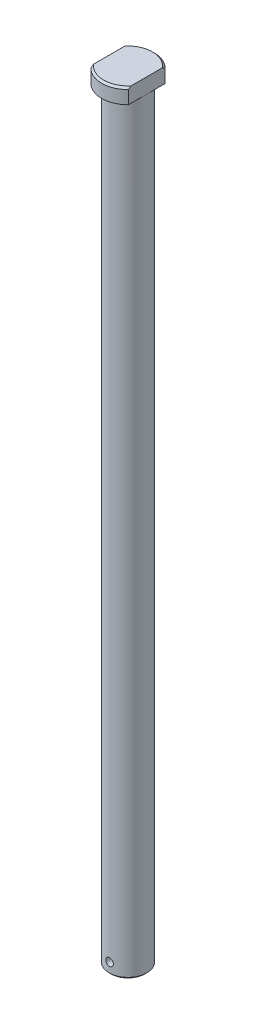
from build123d import *

# Parameters (mm, degrees)
CHAMFER1_SIZE           = 0.5
CUT_EXTRUDE1_DEPTH      = 208.236579783
CUT_EXTRUDE1_DEPTH_BACK = 208.236579783
SKETCH2_R               = 1
CUT_EXTRUDE2_DEPTH      = 208.236579783
CUT_EXTRUDE2_DEPTH_BACK = 208.236579783
SKETCH3_W               = 2
SKETCH3_H               = 4
CUT_EXTRUDE3_DEPTH      = 208.236579783
CUT_EXTRUDE3_DEPTH_BACK = 208.236579783
SKETCH4_W               = 2
SKETCH4_H               = 4


with BuildPart() as part:
    # Sketch1 → Revolve1 (revolve)
    with BuildSketch(Plane.XY):
        Polygon((0, 0), (7, 0), (7, -4), (5, -4), (5, -207), (0, -207), align=None)
    revolve(axis=Axis((0, -318.988143723, 0), (0, 1, 0)))

    # Chamfer1
    chamfer1_edges = [part.edges().sort_by_distance(p)[0] for p in [
        (-5, -207, 0),
        (-7, 0, 0),
    ]]
    chamfer(chamfer1_edges, length=CHAMFER1_SIZE)

    # Sketch2 → Cut-Extrude1 (cut, two sides: drawn at the far end of the back side and taken through both)
    with BuildSketch(Plane.XY.offset(-CUT_EXTRUDE1_DEPTH_BACK)):
        with Locations((0, -204)):
            Circle(SKETCH2_R)
    extrude(amount=CUT_EXTRUDE1_DEPTH + CUT_EXTRUDE1_DEPTH_BACK, mode=Mode.SUBTRACT)

    # Sketch3 → Cut-Extrude2 (cut, two sides: drawn at the far end of the back side and taken through both)
    with BuildSketch(Plane.XY.offset(-CUT_EXTRUDE2_DEPTH_BACK)):
        with Locations((-6, -2)):
            Rectangle(SKETCH3_W, SKETCH3_H)
    extrude(amount=CUT_EXTRUDE2_DEPTH + CUT_EXTRUDE2_DEPTH_BACK, mode=Mode.SUBTRACT)

    # Sketch4 → Cut-Extrude3 (cut, two sides: drawn at the far end of the back side and taken through both)
    with BuildSketch(Plane.XY.offset(-CUT_EXTRUDE3_DEPTH_BACK)):
        with Locations((6, -2)):
            Rectangle(SKETCH4_W, SKETCH4_H)
    extrude(amount=CUT_EXTRUDE3_DEPTH + CUT_EXTRUDE3_DEPTH_BACK, mode=Mode.SUBTRACT)


solid = part.part
